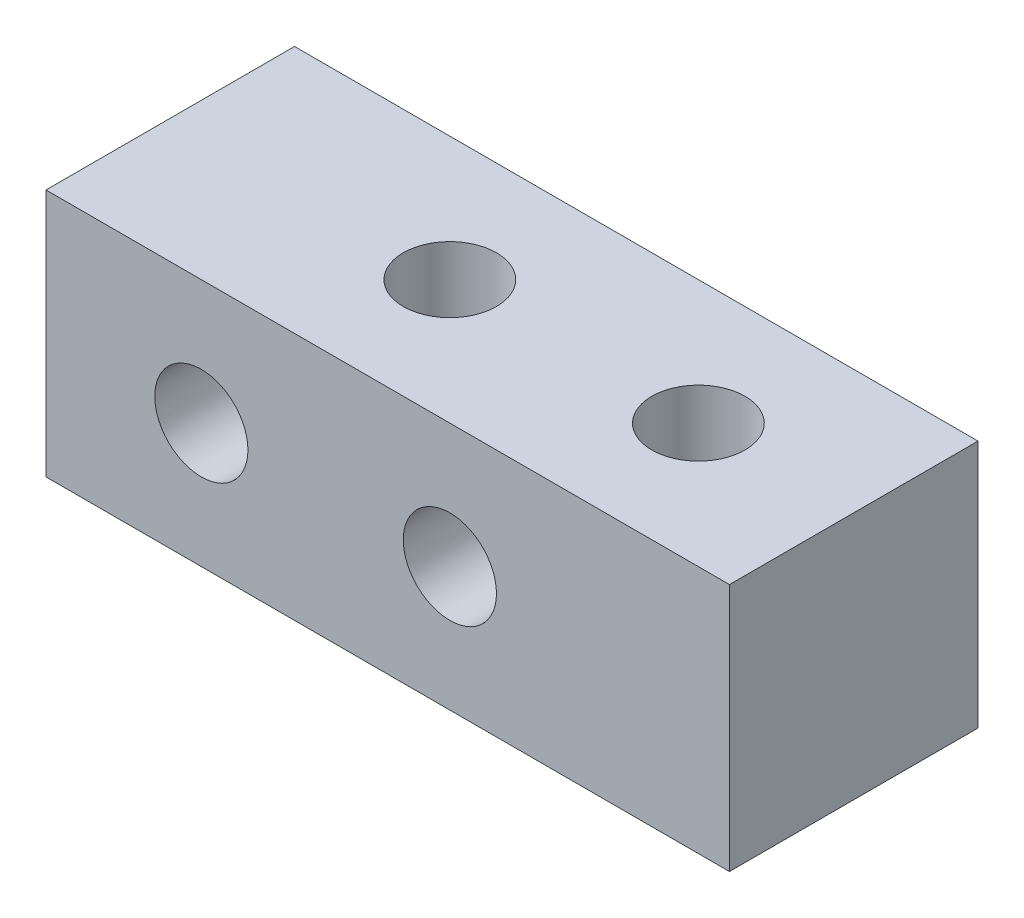
from build123d import *

# Parameters (mm, degrees)
SKETCH_1_W          = 22
SKETCH_1_H          = 8
SKETCH_1_R          = 1.5
EXTRUDE_1_DEPTH     = 8
SKETCH_2_R          = 1.5
CUT_EXTRUDE_1_DEPTH = 16.779733838


with BuildPart() as part:
    # 草图1 → 凸台-拉伸1 (new body)
    with BuildSketch(Plane.XY):
        Rectangle(SKETCH_1_W, SKETCH_1_H)
        with Locations((-6, 0)):
            Circle(SKETCH_1_R, mode=Mode.SUBTRACT)
        with Locations((2, 0)):
            Circle(SKETCH_1_R, mode=Mode.SUBTRACT)
    extrude(amount=EXTRUDE_1_DEPTH)

    # 草图2 → 切除-拉伸1 (cut, through all)
    with BuildSketch(Plane(origin=(0, 4, 0), x_dir=(1, 0, 0), z_dir=(0, 1, 0))):
        with Locations(Location((6, -4, 0), (0, 0, 180))):
            Circle(SKETCH_2_R)
        with Locations(Location((-2, -4, 0), (0, 0, 180))):
            Circle(SKETCH_2_R)
    extrude(amount=-CUT_EXTRUDE_1_DEPTH, mode=Mode.SUBTRACT)


solid = part.part
